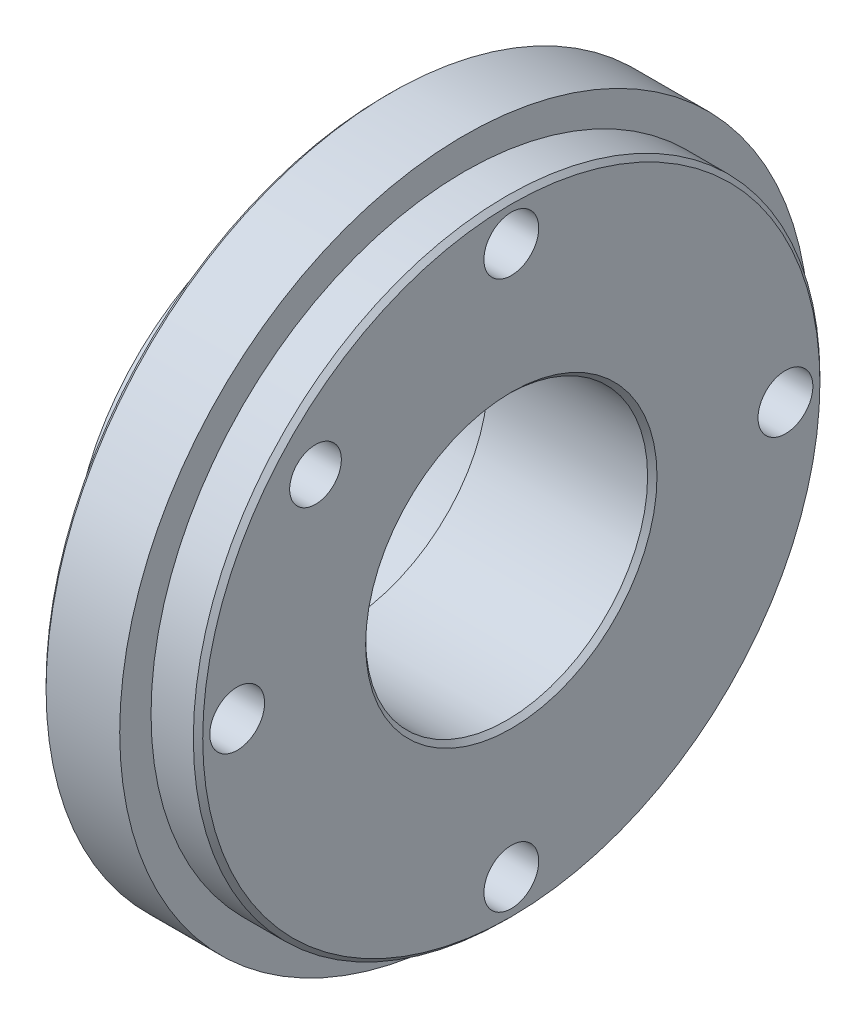
SolidWorks part; units mm, degrees
ref_plane "Front Plane" through (0, 0, 0) normal (0, 0, 1) x (1, 0, 0)
ref_plane "Top Plane" through (0, 0, 0) normal (0, 1, 0) x (1, 0, 0)
ref_plane "Right Plane" through (0, 0, 0) normal (1, 0, 0) x (0, 0, -1)
sketch "Sketch1" plane through (0, 0, 0) normal (0, 0, 1) x (1, 0, 0)
  line L0 (0, 0) -> (32.0465, 0) construction
  line L1 (0, 9) -> (0, 14)
  line L2 (0, 14) -> (15, 14)
  line L3 (15, 14) -> (15, 22)
  line L4 (15, 22) -> (20, 22)
  line L5 (20, 22) -> (20, 9)
  line L8 (0, 9) -> (20, 9)
  point P6 (0, 0)
  dimension "D1" = 9
  dimension "D2" = 14
  dimension "D3" = 22
  dimension "D4" = 5
  dimension "D5" = 15
revolve "Revolve1" add sketch "Sketch1" angle 360 about L0
sketch "Sketch3" plane through (0, 0, 0) normal (0, 0, 1) x (1, 0, 0)
  line L0 (9.6133, 17.5629) -> (8.3867, -17.5629)
  line L1 (8.3867, -17.5629) -> (-5.4157, -17.5629)
  line L2 (-5.4157, -17.5629) -> (-5.4157, 17.5629)
  line L3 (-5.4157, 17.5629) -> (9.6133, 17.5629)
  line L4 (15, 14) -> (15, -14) construction
  line L5 (9, 0) -> (15, 0) construction
  line L6 (15, 22) -> (15, -22) construction
  dimension "D1" = 2
  dimension "D2" = 6
extrude "Cut-Extrude1" cut sketch "Sketch3" against normal mid plane 30
sketch "Sketch4" plane through (8.989, -0.3139, 0) normal (-0.9994, 0.0349, 0) x (0, 0, 1)
  circle A0 centre (0, 0) radius 10.25
  dimension "D1" = 20.5
extrude "Cut-Extrude2" cut sketch "Sketch4" against normal blind 3.5
sketch "Sketch5" plane through (15, 0, 0) normal (-1, 0, 0) x (0, 0, 1)
  line L0 (0, 0) -> (17.5, 0) construction
  line L1 (0, 0) -> (0, 17.5) construction
  line L2 (-17.5, 0) -> (0, 0) construction
  line L3 (0, 0) -> (17.5, 0) construction
  line L4 (0, 0) -> (0, -17.5) construction
  line L5 (0, 0) -> (0, 17.5) construction
  circle A0 centre (0, 0) radius 17.5 construction
  circle A1 centre (-17.5, 0) radius 1.75
  circle A2 centre (0, 17.5) radius 1.75
  circle A3 centre (17.5, 0) radius 1.75
  circle A4 centre (0, -17.5) radius 1.75
  dimension "D1" = 35
  dimension "D2" = 3.5
  dimension "D3" = 90
  dimension "D4" = 0
extrude "Cut-Extrude3" cut sketch "Sketch5" against normal up to surface (5 mm away) up to face at (20, 0, 22)
sketch "Sketch7" plane through (20, 0, 0) normal (1, 0, 0) x (0, 0, -1)
  circle A0 centre (0, 0) radius 20
  circle A1 centre (17.5, 0) radius 1.75 construction
  circle A2 centre (0, -17.5) radius 1.75 construction
  circle A3 centre (-17.5, 0) radius 1.75 construction
  circle A4 centre (0, 17.5) radius 1.75 construction
  circle A5 centre (17.5, 0) radius 1.75
  circle A6 centre (0, -17.5) radius 1.75
  circle A7 centre (-17.5, 0) radius 1.75
  circle A8 centre (0, 17.5) radius 1.75
  circle A9 centre (0, 0) radius 9 construction
  circle A10 centre (0, 0) radius 9
  dimension "D1" = 40
extrude "Boss-Extrude1" add sketch "Sketch7" along normal blind 3
sketch "Sketch10" plane through (23, 0, 0) normal (1, 0, 0) x (0, 0, -1)
  line L0 (0, 0) -> (0, 11) construction
  line L1 (0, 11) -> (-12.5, 11) construction
  circle A0 centre (-12.5, 11) radius 1.65
  dimension "D3" = 3.3
  dimension "D1" = 11
  dimension "D2" = 12.5
extrude "Cut-Extrude5" cut sketch "Sketch10" against normal up to next
cosmetic thread "Cosmetic Thread2" parameters "D2"=4
chamfer "Chamfer1" distance 0.3 angle 45 2 edges at (23, 0, -20) (15, 0, 22)
chamfer "Chamfer2" distance 0.3 angle 45 1 edges at (23, 0, -9)
